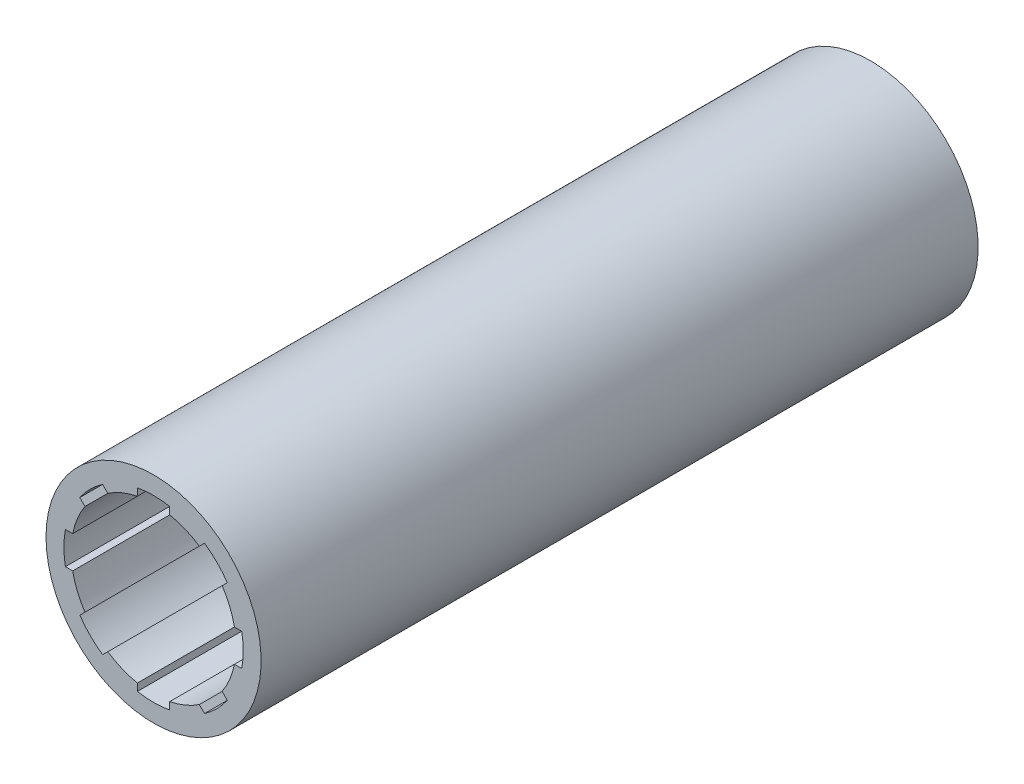
from build123d import *

# Parameters (mm, degrees)
SKETCH_1_R          = 30
EXTRUDE_1_DEPTH     = 100
CUT_EXTRUDE_1_DEPTH = 80
CUT_EXTRUDE_START   = -80
CUT_EXTRUDE_2_DEPTH = 80


with BuildPart() as part:
    # 草图1 → 凸台-拉伸1 (new, symmetric)
    with BuildSketch(Plane.XY):
        with Locations(Location((0, 0, 0), (0, 0, 180))):
            Circle(SKETCH_1_R)
    extrude(amount=EXTRUDE_1_DEPTH, both=True)

    # 草图2 → 切除-拉伸1 (cut)
    with BuildSketch(Plane.XY.offset(100)):
        with BuildLine():
            Line((-4.5, 24.591665255), (-4.5, 22.555487137))
            ThreePointArc((-4.5, 22.555487137), (-8.801718944, 21.249229248), (-12.767157392, 19.131118423))
            Line((-12.767157392, 19.131118423), (-14.206952747, 20.570913778))
            ThreePointArc((-14.206952747, 20.570913778), (-17.67766953, 17.67766953), (-20.570913778, 14.206952747))
            Line((-20.570913778, 14.206952747), (-19.131118423, 12.767157392))
            ThreePointArc((-19.131118423, 12.767157392), (-21.249229248, 8.801718944), (-22.555487137, 4.5))
            Line((-22.555487137, 4.5), (-24.591665255, 4.5))
            ThreePointArc((-24.591665255, 4.5), (-25, 0), (-24.591665255, -4.5))
            Line((-24.591665255, -4.5), (-22.555487137, -4.5))
            ThreePointArc((-22.555487137, -4.5), (-21.249229248, -8.801718944), (-19.131118423, -12.767157392))
            Line((-19.131118423, -12.767157392), (-20.570913778, -14.206952747))
            ThreePointArc((-20.570913778, -14.206952747), (-17.67766953, -17.67766953), (-14.206952747, -20.570913778))
            Line((-14.206952747, -20.570913778), (-12.767157392, -19.131118423))
            ThreePointArc((-12.767157392, -19.131118423), (-8.801718944, -21.249229248), (-4.5, -22.555487137))
            Line((-4.5, -22.555487137), (-4.5, -24.591665255))
            ThreePointArc((-4.5, -24.591665255), (0, -25), (4.5, -24.591665255))
            Line((4.5, -24.591665255), (4.5, -22.555487137))
            ThreePointArc((4.5, -22.555487137), (8.801718944, -21.249229248), (12.767157392, -19.131118423))
            Line((12.767157392, -19.131118423), (14.206952747, -20.570913778))
            ThreePointArc((14.206952747, -20.570913778), (17.67766953, -17.67766953), (20.570913778, -14.206952747))
            Line((20.570913778, -14.206952747), (19.131118423, -12.767157392))
            ThreePointArc((19.131118423, -12.767157392), (21.249229248, -8.801718944), (22.555487137, -4.5))
            Line((22.555487137, -4.5), (24.591665255, -4.5))
            ThreePointArc((24.591665255, -4.5), (25, 0), (24.591665255, 4.5))
            Line((24.591665255, 4.5), (22.555487137, 4.5))
            ThreePointArc((22.555487137, 4.5), (21.249229248, 8.801718944), (19.131118423, 12.767157392))
            Line((19.131118423, 12.767157392), (20.570913778, 14.206952747))
            ThreePointArc((20.570913778, 14.206952747), (17.67766953, 17.67766953), (14.206952747, 20.570913778))
            Line((14.206952747, 20.570913778), (12.767157392, 19.131118423))
            ThreePointArc((12.767157392, 19.131118423), (8.801718944, 21.249229248), (4.5, 22.555487137))
            Line((4.5, 22.555487137), (4.5, 24.591665255))
            ThreePointArc((4.5, 24.591665255), (0, 25), (-4.5, 24.591665255))
        make_face()
    extrude(amount=-CUT_EXTRUDE_1_DEPTH, mode=Mode.SUBTRACT)

    # 草图3 → 切除-拉伸2 (cut)
    with BuildSketch(Plane(origin=(0, 0, -100), x_dir=(-1, 0, 0), z_dir=(0, 0, -1)).offset(CUT_EXTRUDE_START)):
        with BuildLine():
            Line((-4, 22.649503306), (-4, 20.615528128))
            ThreePointArc((-4, 20.615528128), (-8.03635208, 19.401470183), (-11.748952612, 17.405806862))
            Line((-11.748952612, 17.405806862), (-13.187190253, 18.844044503))
            ThreePointArc((-13.187190253, 18.844044503), (-16.263455967, 16.263455967), (-18.844044503, 13.187190253))
            Line((-18.844044503, 13.187190253), (-17.405806862, 11.748952612))
            ThreePointArc((-17.405806862, 11.748952612), (-19.401470183, 8.03635208), (-20.615528128, 4))
            Line((-20.615528128, 4), (-22.649503306, 4))
            ThreePointArc((-22.649503306, 4), (-23, 0), (-22.649503306, -4))
            Line((-22.649503306, -4), (-20.615528128, -4))
            ThreePointArc((-20.615528128, -4), (-19.401470183, -8.03635208), (-17.405806862, -11.748952612))
            Line((-17.405806862, -11.748952612), (-18.844044503, -13.187190253))
            ThreePointArc((-18.844044503, -13.187190253), (-16.263455967, -16.263455967), (-13.187190253, -18.844044503))
            Line((-13.187190253, -18.844044503), (-11.748952612, -17.405806862))
            ThreePointArc((-11.748952612, -17.405806862), (-8.03635208, -19.401470183), (-4, -20.615528128))
            Line((-4, -20.615528128), (-4, -22.649503306))
            ThreePointArc((-4, -22.649503306), (0, -23), (4, -22.649503306))
            Line((4, -22.649503306), (4, -20.615528128))
            ThreePointArc((4, -20.615528128), (8.03635208, -19.401470183), (11.748952612, -17.405806862))
            Line((11.748952612, -17.405806862), (13.187190253, -18.844044503))
            ThreePointArc((13.187190253, -18.844044503), (16.263455967, -16.263455967), (18.844044503, -13.187190253))
            Line((18.844044503, -13.187190253), (17.405806862, -11.748952612))
            ThreePointArc((17.405806862, -11.748952612), (19.401470183, -8.03635208), (20.615528128, -4))
            Line((20.615528128, -4), (22.649503306, -4))
            ThreePointArc((22.649503306, -4), (23, 0), (22.649503306, 4))
            Line((22.649503306, 4), (20.615528128, 4))
            ThreePointArc((20.615528128, 4), (19.401470183, 8.03635208), (17.405806862, 11.748952612))
            Line((17.405806862, 11.748952612), (18.844044503, 13.187190253))
            ThreePointArc((18.844044503, 13.187190253), (16.263455967, 16.263455967), (13.187190253, 18.844044503))
            Line((13.187190253, 18.844044503), (11.748952612, 17.405806862))
            ThreePointArc((11.748952612, 17.405806862), (8.03635208, 19.401470183), (4, 20.615528128))
            Line((4, 20.615528128), (4, 22.649503306))
            ThreePointArc((4, 22.649503306), (0, 23), (-4, 22.649503306))
        make_face()
    extrude(amount=CUT_EXTRUDE_2_DEPTH, mode=Mode.SUBTRACT)


solid = part.part
